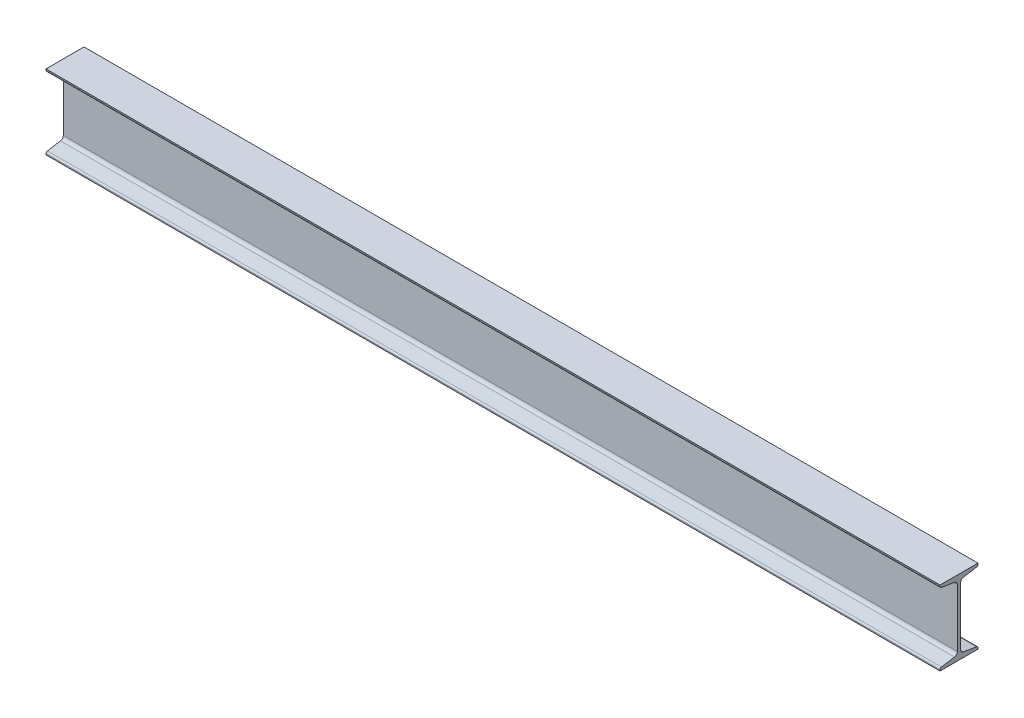
SolidWorks part; units mm, degrees
ref_plane "Front" through (0, 0, 0) normal (0, 0, 1) x (1, 0, 0)
ref_plane "Top" through (0, 0, 0) normal (0, 1, 0) x (1, 0, 0)
ref_plane "Right" through (0, 0, 0) normal (1, 0, 0) x (0, 0, -1)
sketch "Sketch1" plane through (0, 0, 0) normal (1, 0, 0) x (0, 0, -1)
  line L0 (-51, 0) -> (51, 0)
  line L1 (0, 106.3348) -> (0, -35.2641) construction
  line L2 (-4.5, 185.475) -> (-4.5, 14.525)
  line L3 (-4.5, 14.525) -> (-51, 6.775)
  line L4 (-51, 6.775) -> (-51, 0)
  line L5 (-51, 6.775) -> (-4.5, 6.775) construction
  line L6 (-4.5, 6.775) -> (-4.5, 14.525) construction
  line L7 (-23.25, 200) -> (-23.25, 0) construction
  line L8 (-51, 200) -> (51, 200)
  line L9 (-51, 200) -> (-51, 193.225)
  line L10 (-51, 193.225) -> (-4.5, 185.475)
  line L11 (-51, 193.225) -> (-4.5, 193.225) construction
  line L12 (-4.5, 193.225) -> (-4.5, 185.475) construction
  line L13 (-23.25, 11.4) -> (-23.25, 0) construction
  line L14 (-23.25, 200) -> (-23.25, 188.6) construction
  line L15 (51, 6.775) -> (51, 0)
  line L16 (4.5, 14.525) -> (51, 6.775)
  line L17 (4.5, 185.475) -> (4.5, 14.525)
  line L18 (51, 193.225) -> (4.5, 185.475)
  line L19 (51, 200) -> (51, 193.225)
  point P22 (0, 200)
extrude "Base" add sketch "Sketch1" along normal blind 2400
fillet "Fillet1" radius 9 4 edges at (1200, 185.475, -4.5) (1200, 14.525, -4.5) (1200, 14.525, 4.5) (1200, 185.475, 4.5)
fillet "Fillet2" radius 4.5 4 edges at (1200, 193.225, 51) (1200, 6.775, 51) (1200, 6.775, -51) (1200, 193.225, -51)
equation "\"D5@Sketch1\" =  ( \"b@Sketch1\" - \"d@Sketch1\" ) /12"
equation "\"D10@Sketch1\" = \"D5@Sketch1\""
equation "\"t1@Sketch1\" = \"t@Sketch1\""
equation "\"D6@Sketch1\" =  ( \"b@Sketch1\" - \"d@Sketch1\" ) /4"
